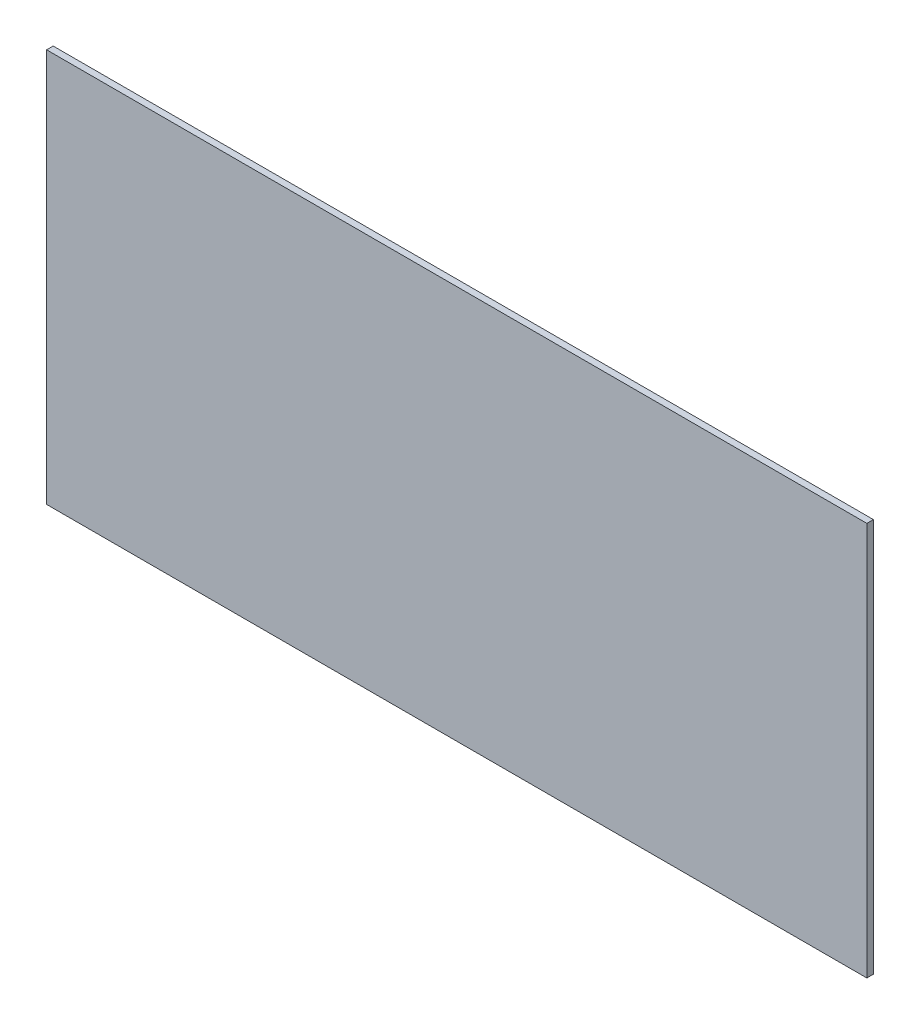
from build123d import *

# Parameters (mm, degrees)
SKETCH1_W           = 250
SKETCH1_H           = 120
BOSS_EXTRUDE1_DEPTH = 2


with BuildPart() as part:
    # Sketch1 → Boss-Extrude1 (new body)
    with BuildSketch(Plane.XY):
        with Locations((125, 60)):
            Rectangle(SKETCH1_W, SKETCH1_H)
    extrude(amount=BOSS_EXTRUDE1_DEPTH)


solid = part.part
